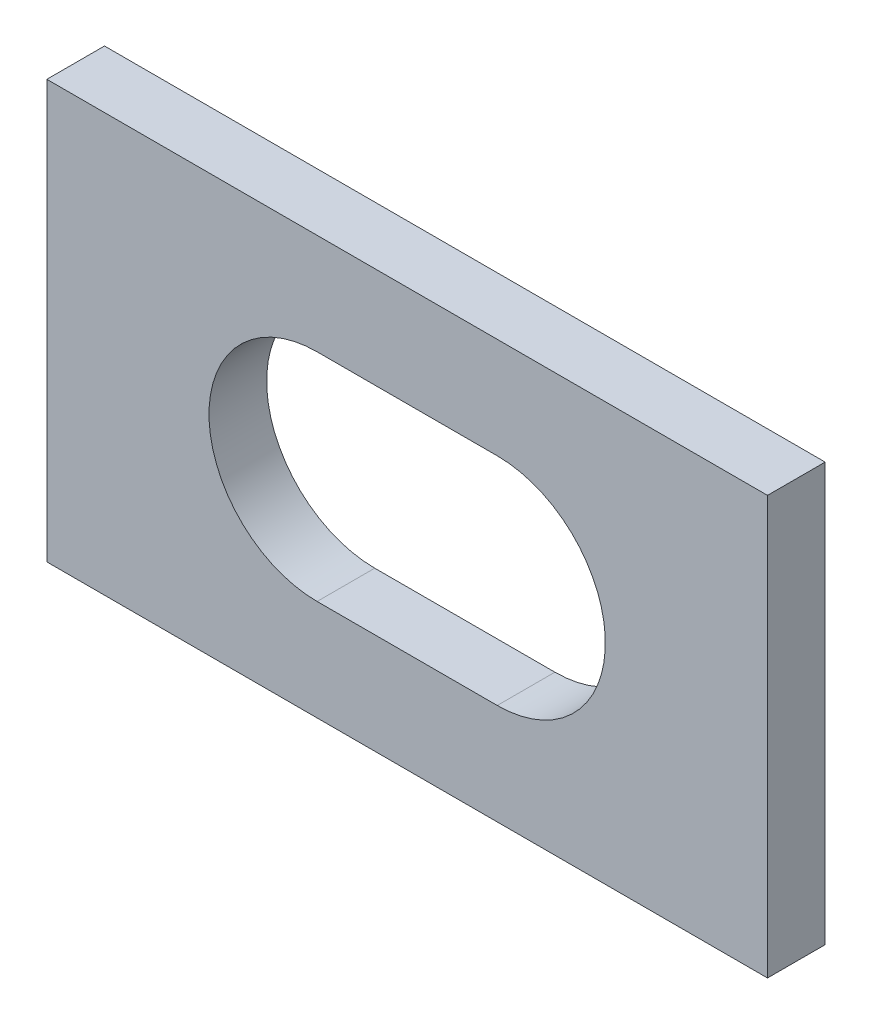
from build123d import *

# Parameters (mm, degrees)
SKETCH1_W           = 200
SKETCH1_H           = 116
BOSS_EXTRUDE1_DEPTH = 16


with BuildPart() as part:
    # Sketch1 → Boss-Extrude1 (new body)
    with BuildSketch(Plane.XY):
        with Locations((25, 0)):
            Rectangle(SKETCH1_W, SKETCH1_H)
        with BuildLine():
            Line((0, 30), (50, 30))
            ThreePointArc((50, 30), (80, 0), (50, -30))
            Line((50, -30), (0, -30))
            ThreePointArc((0, -30), (-30, 0), (0, 30))
        make_face(mode=Mode.SUBTRACT)
    extrude(amount=BOSS_EXTRUDE1_DEPTH)


solid = part.part
